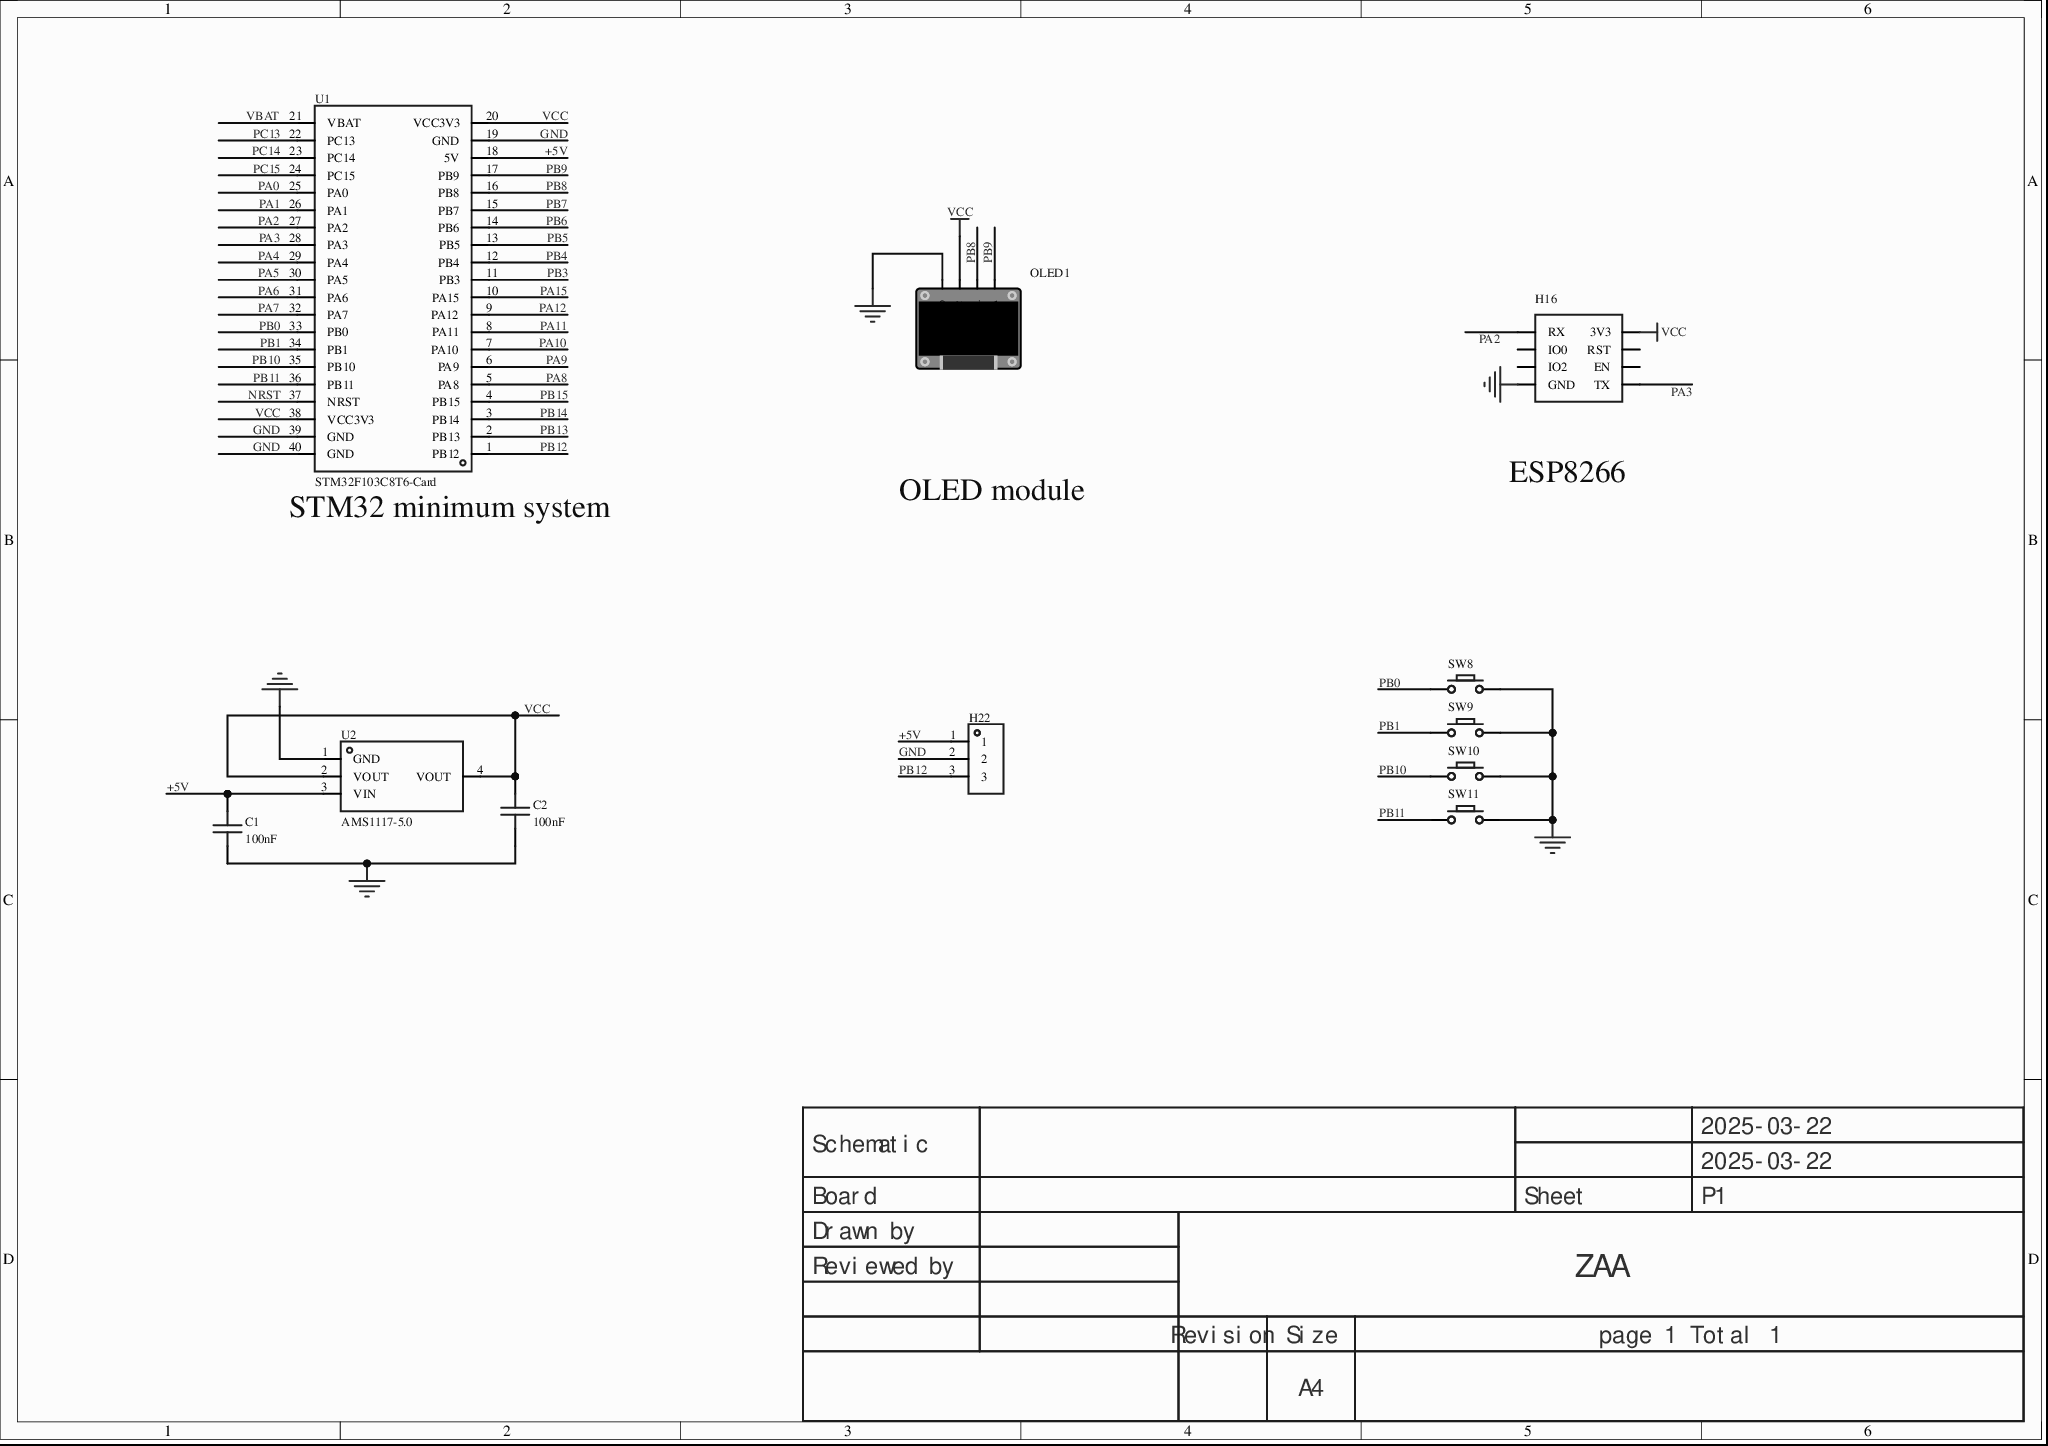
[diagram p0: MISC89072-3.schdoc]
# Altium project MISC89072-2.PrjPcb
1 sheet, 11 parts. Net scope: global (net labels, ports and power ports of the same name join across sheets).
Board file: MISC89072.pcbdoc

## Sheet MISC89072-3.schdoc
size 297 x 209 mm; Version: V1.0; @Project Name: MISC89072; @Page Count: 1; @Update Date: 2025-03-22; @Create Date: 2025-03-22; @Schematic Name: MISC89072; @Page No: 1; @Create Time: 17:30:36; @Update Time: 17:30:49; @Board Name: MISC89072

### Parts
C1  100nF  [C0603]
C2  100nF  [C0603]
H16  (no value)  [HDR-TH_8P-P2.54-V-F-R2-C4-S2.54-1]
H22  (no value)  [HDR-TH_3P-P2.54-V-F]
OLED1  (no value)  [0.96OLED_4P]
SW8  (no value)  [Key_TH_3.5x6x4.3]
SW9  (no value)  [Key_TH_3.5x6x4.3]
SW10  (no value)  [Key_TH_3.5x6x4.3]
SW11  (no value)  [Key_TH_3.5x6x4.3]
U1  STM32F103C8T6-Card  [CONN-TH_L53.3-W22.9_STM32F103C8T6-CARD]
U2  AMS1117-5.0  [SOT-223_L6.5-W3.5-P2.30-LS7.0-BR]

### Nets
GND: C1.1 C2.1 H16.2(GND) H22.2 OLED1.1(GND) SW8.B SW9.B SW10.B SW11.B U1.19(GND) U1.39(GND) U1.40(GND) U2.1(GND)
VCC: C2.2 H16.7(3V3) OLED1.2(VCC) U1.20(VCC3V3) U1.38(VCC3V3) U2.2(VOUT) U2.4(VOUT)
+5V: C1.2 H22.1 U1.18(5V) U2.3(VIN)
NRST: U1.37(NRST)
PA0: U1.25(PA0)
PA1: U1.26(PA1)
PA2: H16.8(RX) U1.27(PA2)
PA3: H16.1(TX) U1.28(PA3)
PA4: U1.29(PA4)
PA5: U1.30(PA5)
PA6: U1.31(PA6)
PA7: U1.32(PA7)
PA8: U1.5(PA8)
PA9: U1.6(PA9)
PA10: U1.7(PA10)
PA11: U1.8(PA11)
PA12: U1.9(PA12)
PA15: U1.10(PA15)
PB0: SW8.A U1.33(PB0)
PB1: SW9.A U1.34(PB1)
PB3: U1.11(PB3)
PB4: U1.12(PB4)
PB5: U1.13(PB5)
PB6: U1.14(PB6)
PB7: U1.15(PB7)
PB8: OLED1.3(SCL) U1.16(PB8)
PB9: OLED1.4(SDA) U1.17(PB9)
PB10: SW10.A U1.35(PB10)
PB11: SW11.A U1.36(PB11)
PB12: H22.3 U1.1(PB12)
PB13: U1.2(PB13)
PB14: U1.3(PB14)
PB15: U1.4(PB15)
PC13: U1.22(PC13)
PC14: U1.23(PC14)
PC15: U1.24(PC15)
VBAT: U1.21(VBAT)

Not connected (* = marked no-connect by the designer): H16 3(EN) 4(IO2) 5(RST) 6(IO0)

### Notes on the sheet
- (near U1) STM32 minimum system
- OLED module
- ESP8266
- 2025-03-22
- Schematic
- Board
- Sheet
- P1
- Drawn by
- Reviewed by
- ZAA
- Revision
- Size
- A4
- page 1 Total 1

### Library data of the parts
C1 C2 = CAP_0603: ConvertToPcb: yes; SymbolName: CapAcitance; ModelId: ac125912035d415993ca9572d50418b1; ModelName: C0603_L1.6-W0.8-H0.8; ModelTransform: 62.992,31.496,0,0,0,0,0,0,0; Device: CAP_0603; AddInBom: yes; Supplier Footprint: 0603; FootprintName: C0603; Value: 100nF
H16 = HDR-F_2.54_2x4: ConvertToPcb: yes; SymbolName: HDR-F-2.54_2x4; ModelId: 64729f32a5874cf59655d275a66f1050; ModelName: HDR2.54-F-LI-2X4P; ModelTransform: 399.999,200,0,0,0,0,0,0,-118.11; Device: HDR-F_2.54_2x4; AddInBom: yes; SupplierPart: C92271; Supplier Footprint: 插件; FootprintName: HDR-TH_8P-P2.54-V-F-R2-C4-S2.54-1
H22 = HDR-F_2.54_1x3P: Symbol: PM254V-11-03-H85; ConvertToPcb: yes; ModelId: f3b3cc5aae9641bf9e56fc160cef875b; ModelName: HDR2.54-F-LI-1X3P; ModelTransform: 299.9994,100,0,0,0,0,0,0,-118.11; Device: HDR-F_2.54_1x3P; AddInBom: yes; SupplierPart: C541850; Supplier Footprint: 插件; FootprintName: HDR-TH_3P-P2.54-V-F
OLED1 = 0.96OLED模块_4P: Device: 0.96OLED module_4P; ConvertToPcb: yes; ModelId: 79c000fdb68d45a296c2e9bedf4f9055; ModelTransform: 1393.69792,1318.895,0,0,0,0,0,-560.079,-137.795; AddInBom: yes; SymbolName: 0.96OLED module_4P; FootprintName: 0.96OLED_4P; Supplier Footprint: 插件; ModelName: 0.96OLED_4P
SW8-SW11 = Key_TH_3.5x6x4.3: ConvertToPcb: yes; ModelId: c3523f9014d949d7ba5445190a3178990819f05c4eef4c71ace90d822a990e87; ModelName: SW-TH_L6.0-W3.5-H5.0-P6.5; ModelTransform: 308.49,137.8,335.08,0,0,0,0,0,-129.92; Device: Key_TH_3.5x6x4.3; AddInBom: yes; Supplier Footprint: 插件; SymbolName: Key_TH_3.5x6x4.3; FootprintName: Key_TH_3.5x6x4.3
U1 = STM32F103C8T6-Card: AddInBom: yes; Symbol: STM32F103C8T6-CARD; Device: STM32F103C8T6-Card; LCSC Part Name: STM32F103C8T6-Card; SupplierPart: C9900077949; ManufacturerPart: STM32F103C8T6-Card; Supplier Footprint: 插件; Supplier: LCSC; ConvertToPcb: yes; FootprintName: CONN-TH_L53.3-W22.9_STM32F103C8T6-CARD
U2 = AMS1117-5.0_C6187: 输出类型:固定;工作电压:12V;输出电压:5V;输出电流:1A;电源纹波抑制比(PSRR):-;输出极性:正极;; Manufacturer: AMS; AddInBom: yes; ModelId: 925194bf9823436183a3e0b978a8d076; ModelName: SOT-223-4P_L6.5-W3.5-H1.6-LS7.0-P2.30; ModelTransform: 279.89794,255.905,0,180,0,0,0.0005,0.0005,0; Output Type: Fixed; Voltage - Supply: 12V; Output Voltage: 5V; Output Current: 1A; Voltage Dropout: 1.3V@(1A); Output Configuration: Positive; Number of Outputs: 1; Symbol: AMS1117-5.0; Device: AMS1117-5.0_C6187; LCSC Part Name: 输入12V 输出5V 1A; SupplierPart: C6187; ManufacturerPart: AMS1117-5.0; Supplier Footprint: SOT-223; Datasheet: https://atta.szlcsc.com/upload/public/pdf/source/20230918/E4B716057EE82179D88E8A0894830D59.pdf; Supplier: LCSC; ConvertToPcb: yes; FootprintName: SOT-223_L6.5-W3.5-P2.30-LS7.0-BR; Power Supply Rejection Ratio (PSRR): -; standby current: -; Noise: -; Features: Overcurrent protection (OCP); Operating Temperature: -